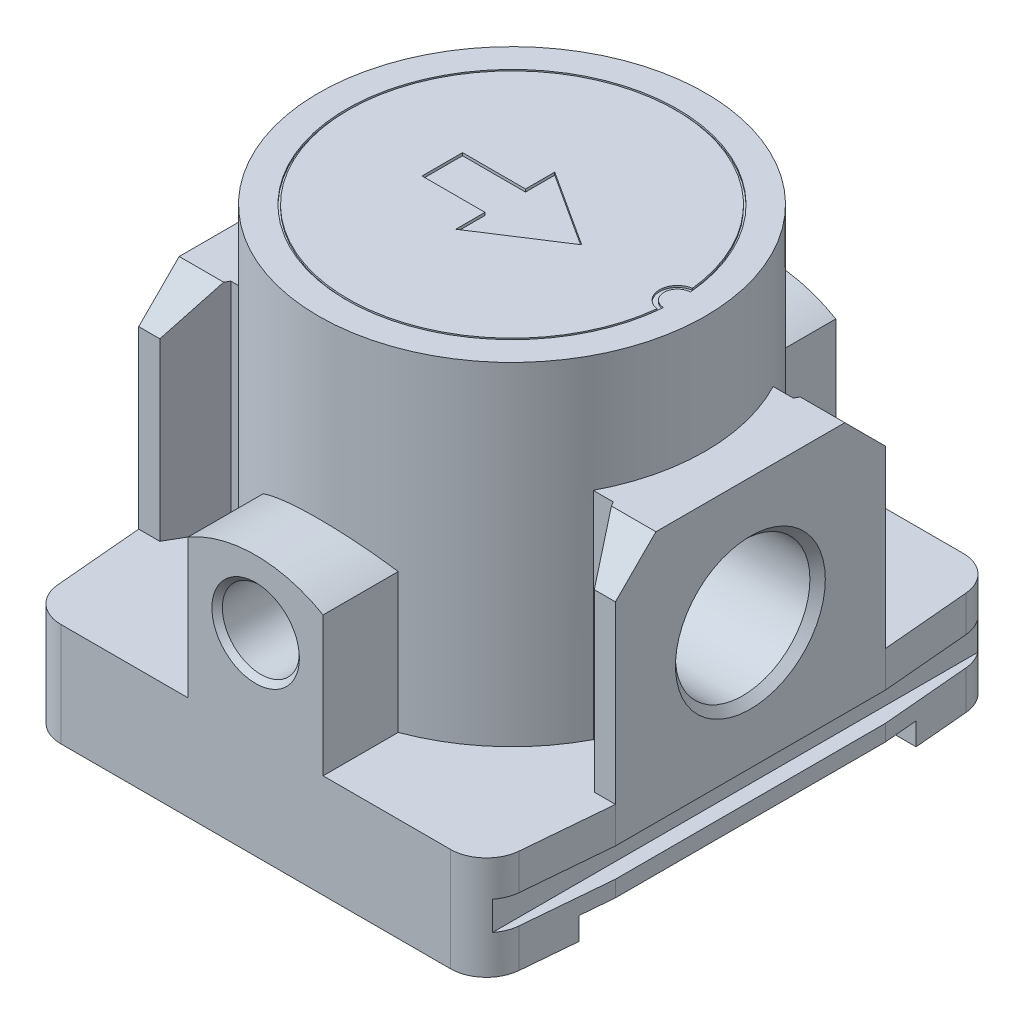
from build123d import *

# Parameters (mm, degrees)
EXTRUDE_1_DEPTH           = 26.5
EXTRUDE_1_DEPTH_BACK      = 26.5
SKETCH_2_W                = 57
SKETCH_2_H                = 61
CUT_EXTRUDE_1_DEPTH       = 21.5
SKETCH_3_W                = 57
SKETCH_3_H                = 34
CUT_EXTRUDE_2_DEPTH       = 24
EXTRUDE_2_DEPTH           = 28.5
EXTRUDE_2_DEPTH_BACK      = 28.5
SKETCH_5_W                = 21.5
SKETCH_5_H                = 37
CUT_EXTRUDE_3_DEPTH       = 28.5
CUT_EXTRUDE_3_DEPTH_BACK  = 28.5
SKETCH_6_W                = 1.7
SKETCH_6_H                = 3.2
CUT_EXTRUDE_4_DEPTH       = 28.5
CUT_EXTRUDE_4_DEPTH_BACK  = 28.5
SKETCH_7_W                = 1.7
SKETCH_7_H                = 3.2
HOLE_WIZARD_1_D           = 8.566
HOLE_WIZARD_1_DEPTH       = 8.2
HOLE_WIZARD_1_CSINK_D     = 9.728
HOLE_WIZARD_1_CSINK_ANGLE = 90
HOLE_WIZARD_1_TIP         = 2.472791203
CUT_EXTRUDE_5_DEPTH       = 1.5
HOLE_WIZARD_2_D           = 14.95
HOLE_WIZARD_2_DEPTH       = 11.7
HOLE_WIZARD_2_CSINK_D     = 16.662
HOLE_WIZARD_2_CSINK_ANGLE = 90
HOLE_WIZARD_2_TIP         = 4.315693262
HOLE_WIZARD_3_D           = 14.95
HOLE_WIZARD_3_DEPTH       = 11.7
HOLE_WIZARD_3_CSINK_D     = 16.662
HOLE_WIZARD_3_CSINK_ANGLE = 90
HOLE_WIZARD_3_TIP         = 4.315693262
CUT_EXTRUDE_6_DEPTH       = 0.3
CUT_EXTRUDE_7_DEPTH       = 0.2


with BuildPart() as part:
    # 草图1 → 凸台-拉伸1 (new, two sides: drawn at the far end of the back side and taken through both)
    with BuildSketch(Plane(origin=(0, 0, 0), x_dir=(0, 0, -1), z_dir=(1, 0, 0)).offset(-EXTRUDE_1_DEPTH_BACK)):
        Polygon((-28.5, -21.5), (-18.75, -21.5), (-18.75, -19), (18.75, -19), (18.75, -21.5), (28.5, -21.5), (28.5, -10), (15, -10), (15, 9.5), (10.5, 14), (-10.5, 14), (-15, 9.5), (-15, -10), (-28.5, -10), align=None)
    extrude(amount=EXTRUDE_1_DEPTH + EXTRUDE_1_DEPTH_BACK)

    # 草图2 → 切除-拉伸1 (cut)
    with BuildSketch(Plane(origin=(0, 0, 0), x_dir=(1, 0, 0), z_dir=(0, 1, 0))):
        Rectangle(SKETCH_2_W, SKETCH_2_H)
        with BuildLine():
            Line((-26.5, -15), (-25.638357139, -24.848622971))
            ThreePointArc((-25.638357139, -24.848622971), (-24.355939177, -27.449109347), (-21.653578346, -28.5))
            Line((-21.653578346, -28.5), (21.653578346, -28.5))
            ThreePointArc((21.653578346, -28.5), (24.355939177, -27.449109347), (25.638357139, -24.848622971))
            Line((25.638357139, -24.848622971), (26.5, -15))
            Line((26.5, -15), (26.5, 15))
            Line((26.5, 15), (25.638357139, 24.848622971))
            ThreePointArc((25.638357139, 24.848622971), (24.355939177, 27.449109347), (21.653578346, 28.5))
            Line((21.653578346, 28.5), (-21.653578346, 28.5))
            ThreePointArc((-21.653578346, 28.5), (-24.355939177, 27.449109347), (-25.638357139, 24.848622971))
            Line((-25.638357139, 24.848622971), (-26.5, 15))
            Line((-26.5, 15), (-26.5, -15))
        make_face(mode=Mode.SUBTRACT)
    extrude(amount=-CUT_EXTRUDE_1_DEPTH, mode=Mode.SUBTRACT)

    # 草图3 → 切除-拉伸2 (cut)
    with BuildSketch(Plane(origin=(0, -10, 0), x_dir=(1, 0, 0), z_dir=(0, 1, 0))):
        Rectangle(SKETCH_3_W, SKETCH_3_H)
        Polygon((-26.5, -15), (-24.15, -15), (-21.263248654, -10), (21.263248654, -10), (24.15, -15), (26.5, -15), (26.5, 15), (24.15, 15), (21.263248654, 10), (-21.263248654, 10), (-24.15, 15), (-26.5, 15), align=None, mode=Mode.SUBTRACT)
    extrude(amount=CUT_EXTRUDE_2_DEPTH, mode=Mode.SUBTRACT)

    # 草图4 → 凸台-拉伸2 (add, two sides: drawn at the far end of the back side and taken through both)
    with BuildSketch(Plane.XY.offset(-EXTRUDE_2_DEPTH_BACK)):
        with BuildLine():
            Line((-7.5, -10), (7.5, -10))
            Line((7.5, -10), (7.5, 5.490381057))
            ThreePointArc((7.5, 5.490381057), (0, 7.5), (-7.5, 5.490381057))
            Line((-7.5, 5.490381057), (-7.5, -10))
        make_face()
    extrude(amount=EXTRUDE_2_DEPTH + EXTRUDE_2_DEPTH_BACK)

    # 草图5 → 旋转1 (revolve)
    with BuildSketch(Plane.XY, mode=Mode.PRIVATE) as revolve_1_sk:
        with Locations((10.75, 8.5)):
            Rectangle(SKETCH_5_W, SKETCH_5_H)
    revolve(revolve_1_sk.sketch.rotate(Axis((0, -10, 0), (0, 1, 0)), 270), axis=Axis((0, -10, 0), (0, 1, 0)))

    # 草图6 → 切除-拉伸3 (cut, two sides: drawn at the far end of the back side and taken through both)
    with BuildSketch(Plane.XY.offset(-CUT_EXTRUDE_3_DEPTH_BACK)):
        with Locations((25.65, -15.6)):
            Rectangle(SKETCH_6_W, SKETCH_6_H)
    extrude(amount=CUT_EXTRUDE_3_DEPTH + CUT_EXTRUDE_3_DEPTH_BACK, mode=Mode.SUBTRACT)

    # 草图7 → 切除-拉伸4 (cut, two sides: drawn at the far end of the back side and taken through both)
    with BuildSketch(Plane.XY.offset(-CUT_EXTRUDE_4_DEPTH_BACK)):
        with Locations((-25.65, -15.6)):
            Rectangle(SKETCH_7_W, SKETCH_7_H)
    extrude(amount=CUT_EXTRUDE_4_DEPTH + CUT_EXTRUDE_4_DEPTH_BACK, mode=Mode.SUBTRACT)

    # 草图8 → 切除-旋转1 (revolve, cut)
    with BuildSketch(Plane(origin=(0, 0, 0), x_dir=(1, 0, 0), z_dir=(0, 1, 0)), mode=Mode.PRIVATE) as cut_revolve_1_sk:
        Polygon((4.3, 28.5), (4.3, 27.7), (5.1, 28.5), align=None)
    revolve(cut_revolve_1_sk.sketch.rotate(Axis((0, 0, -27.7), (0, 0, -1)), 180), axis=Axis((0, 0, -27.7), (0, 0, -1)), mode=Mode.SUBTRACT)

    # 孔1
    with Locations(Plane.XY.offset(28.5)):
        with Locations((0, 0)):
            CounterSinkHole(HOLE_WIZARD_1_D / 2, HOLE_WIZARD_1_CSINK_D / 2, depth=HOLE_WIZARD_1_DEPTH, counter_sink_angle=HOLE_WIZARD_1_CSINK_ANGLE)
            with Locations((0, 0, -(HOLE_WIZARD_1_DEPTH + HOLE_WIZARD_1_TIP / 2))):  # 120° drill point
                Cone(0, HOLE_WIZARD_1_D / 2, HOLE_WIZARD_1_TIP, mode=Mode.SUBTRACT)

    # 草图11 → 切除-拉伸5 (cut)
    with BuildSketch(Plane.XY.offset(-28.5)):
        Polygon((-2, 1.154700538), (-2, -1.154700538), (0, -2.309401077), (2, -1.154700538), (2, 1.154700538), (0, 2.309401077), align=None)
    extrude(amount=CUT_EXTRUDE_5_DEPTH, mode=Mode.SUBTRACT)

    # 孔2
    with Locations(Plane(origin=(26.5, 0, 0), x_dir=(0, 0, -1), z_dir=(1, 0, 0))):
        with Locations((0, 0)):
            CounterSinkHole(HOLE_WIZARD_2_D / 2, HOLE_WIZARD_2_CSINK_D / 2, depth=HOLE_WIZARD_2_DEPTH, counter_sink_angle=HOLE_WIZARD_2_CSINK_ANGLE)
            with Locations((0, 0, -(HOLE_WIZARD_2_DEPTH + HOLE_WIZARD_2_TIP / 2))):  # 120° drill point
                Cone(0, HOLE_WIZARD_2_D / 2, HOLE_WIZARD_2_TIP, mode=Mode.SUBTRACT)

    # 孔3
    with Locations(Plane.ZY.offset(26.5)):
        with Locations((0, 0)):
            CounterSinkHole(HOLE_WIZARD_3_D / 2, HOLE_WIZARD_3_CSINK_D / 2, depth=HOLE_WIZARD_3_DEPTH, counter_sink_angle=HOLE_WIZARD_3_CSINK_ANGLE)
            with Locations((0, 0, -(HOLE_WIZARD_3_DEPTH + HOLE_WIZARD_3_TIP / 2))):  # 120° drill point
                Cone(0, HOLE_WIZARD_3_D / 2, HOLE_WIZARD_3_TIP, mode=Mode.SUBTRACT)

    # 草图16 → 切除-拉伸6 (cut)
    with BuildSketch(Plane(origin=(0, 27, 0), x_dir=(1, 0, 0), z_dir=(0, 1, 0))):
        Polygon((-7.75, -2.25), (-0.75, -2.25), (-0.75, -5.5), (7.75, 0), (-0.75, 5.5), (-0.75, 2.25), (-7.75, 2.25), align=None)
    extrude(amount=-CUT_EXTRUDE_6_DEPTH, mode=Mode.SUBTRACT)

    # 草图17 → 切除-拉伸7 (cut)
    with BuildSketch(Plane(origin=(0, 27, 0), x_dir=(1, 0, 0), z_dir=(0, 1, 0))):
        with BuildLine():
            ThreePointArc((18.338858696, 1.498753396), (-18.4, 0), (18.338858696, -1.498753396))
            ThreePointArc((18.338858696, -1.498753396), (16.9, 0), (18.338858696, 1.498753396))
        make_face()
        with BuildLine():
            ThreePointArc((18.092391304, 1.976202644), (-18.2, 0), (18.092391304, -1.976202644))
            ThreePointArc((18.092391304, -1.976202644), (16.4, 0), (18.092391304, 1.976202644))
        make_face(mode=Mode.SUBTRACT)
    extrude(amount=-CUT_EXTRUDE_7_DEPTH, mode=Mode.SUBTRACT)


solid = part.part
